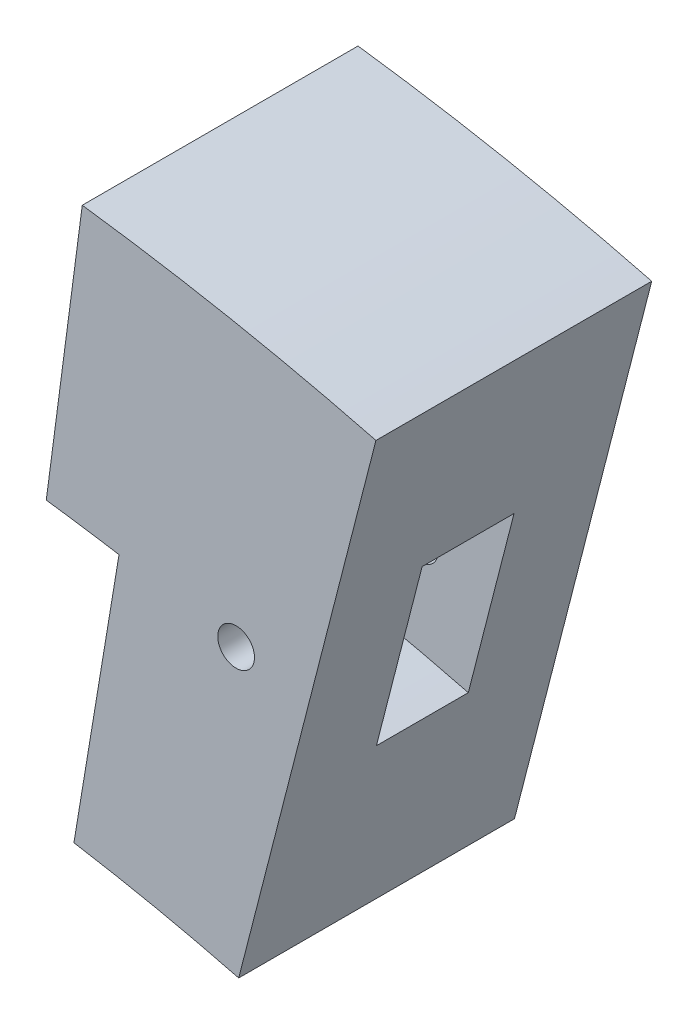
from build123d import *

# Parameters (mm, degrees)
BOSS_EXTRUDE1_DEPTH = 15
CUT_EXTRUDE1_START  = -10
CUT_EXTRUDE1_DEPTH  = 10
BOSS_EXTRUDE3_START = -5
BOSS_EXTRUDE3_DEPTH = 5
SKETCH5_R           = 1
CUT_EXTRUDE2_DEPTH  = 15
CUT_EXTRUDE4_START  = -15
CUT_EXTRUDE4_DEPTH  = 15
CUT_EXTRUDE5_START  = -15
CUT_EXTRUDE5_DEPTH  = 15


with BuildPart() as part:
    # Sketch1 → Boss-Extrude1 (new body)
    with BuildSketch(Plane.XY):
        with BuildLine():
            Line((6.964115375, 114.788941528), (9.188776982, 134.686919846))
            ThreePointArc((9.188776982, 134.686919846), (21.482610172, 133.279771384), (33.595955959, 130.752865143))
            Line((33.595955959, 130.752865143), (26.130187968, 101.696672889))
            ThreePointArc((26.130187968, 101.696672889), (21.669371251, 102.739662982), (17.167305653, 103.587082286))
            Line((17.167305653, 103.587082286), (18.802287144, 113.452518695))
            ThreePointArc((18.802287144, 113.452518695), (12.90051864, 114.274129263), (6.964115375, 114.788941528))
        make_face()
    extrude(amount=BOSS_EXTRUDE1_DEPTH)

    # Sketch3 → Cut-Extrude1 (cut)
    with BuildSketch(Plane.XY.offset(15).offset(CUT_EXTRUDE1_START)):
        with BuildLine():
            ThreePointArc((18.802287144, 113.452518695), (23.733120893, 112.52439279), (28.618777298, 111.382070307))
            Line((28.618777298, 111.382070307), (31.107147965, 121.066616705))
            ThreePointArc((31.107147965, 121.066616705), (19.677605268, 123.440561348), (8.076446178, 124.737930687))
            Line((8.076446178, 124.737930687), (6.964115375, 114.788941528))
            ThreePointArc((6.964115375, 114.788941528), (12.90051864, 114.274129263), (18.802287144, 113.452518695))
        make_face()
    extrude(amount=CUT_EXTRUDE1_DEPTH, mode=Mode.SUBTRACT)

    # Sketch4 → Boss-Extrude3 (add)
    with BuildSketch(Plane.XY.offset(15).offset(BOSS_EXTRUDE3_START)):
        with BuildLine():
            ThreePointArc((28.618777298, 111.382070307), (17.872807715, 113.602652893), (6.964115375, 114.788941528))
            Line((6.964115375, 114.788941528), (8.076446178, 124.737930687))
            ThreePointArc((8.076446178, 124.737930687), (19.677605268, 123.440561348), (31.107147965, 121.066616705))
            Line((31.107147965, 121.066616705), (28.618777298, 111.382070307))
        make_face()
    extrude(amount=BOSS_EXTRUDE3_DEPTH)

    # Sketch5 → Cut-Extrude2 (cut)
    with BuildSketch(Plane.XY.offset(15)):
        with Locations((25.988912996, 117.220204748)):
            Circle(SKETCH5_R)
    extrude(amount=-CUT_EXTRUDE2_DEPTH, mode=Mode.SUBTRACT)

    # Sketch7 → Cut-Extrude4 (cut)
    with BuildSketch(Plane.XY.offset(15).offset(CUT_EXTRUDE4_START)):
        with BuildLine():
            Line((0, 115), (0, 135))
            ThreePointArc((0, 135), (8.829422446, 134.710954637), (17.62103595, 133.845056285))
            Line((17.62103595, 133.845056285), (15.010512105, 114.016159058))
            ThreePointArc((15.010512105, 114.016159058), (7.521359861, 114.753776172), (0, 115))
        make_face()
    extrude(amount=CUT_EXTRUDE4_DEPTH, mode=Mode.SUBTRACT)

    # Sketch8 → Cut-Extrude5 (cut)
    with BuildSketch(Plane.XY.offset(15).offset(CUT_EXTRUDE5_START)):
        with BuildLine():
            Line((15.010512105, 114.016159058), (15.663143066, 118.973383365))
            ThreePointArc((15.663143066, 118.973383365), (17.643911325, 118.695797706), (19.619777889, 118.385236899))
            Line((19.619777889, 118.385236899), (18.802287144, 113.452518695))
            ThreePointArc((18.802287144, 113.452518695), (16.908748354, 113.750139469), (15.010512105, 114.016159058))
        make_face()
    extrude(amount=CUT_EXTRUDE5_DEPTH, mode=Mode.SUBTRACT)


solid = part.part
